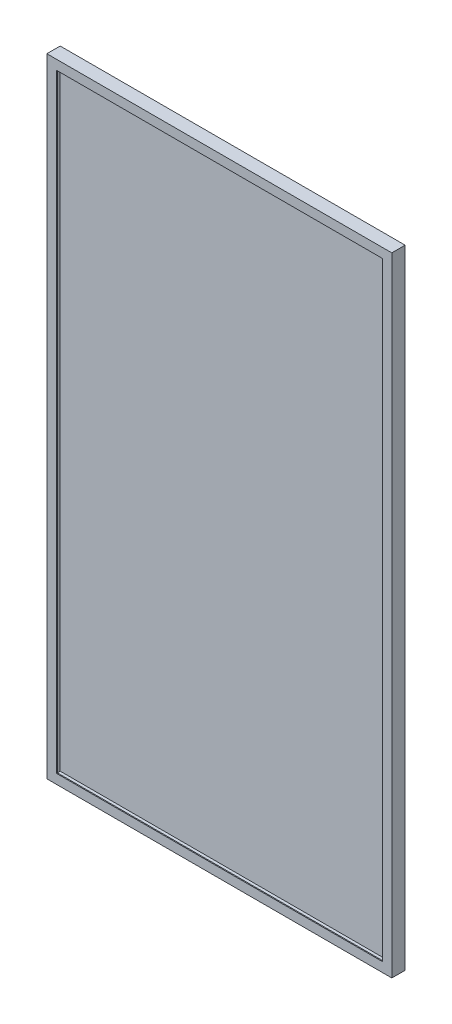
SolidWorks part; units mm, degrees
ref_plane "前视基准面" through (0, 0, 0) normal (0, 0, 1) x (1, 0, 0)
ref_plane "上视基准面" through (0, 0, 0) normal (0, 1, 0) x (1, 0, 0)
ref_plane "右视基准面" through (0, 0, 0) normal (1, 0, 0) x (0, 0, -1)
sketch "草图1" plane through (0, 0, 0) normal (0, 0, 1) x (1, 0, 0)
  line L1 (0, 0) -> (724.5, 0)
  line L2 (0, 0) -> (0, 1319)
  line L3 (0, 1319) -> (724.5, 1319)
  line L4 (724.5, 0) -> (724.5, 1319)
  dimension "D1" = 1319
  dimension "D2" = 724.5
extrude "凸台-拉伸1" add sketch "草图1" along normal blind 28
shell "抽壳1" thickness 2
sketch "草图2" plane through (0, 0, 28) normal (0, 0, 1) x (1, 0, 0)
  line L14 (20, 1299) -> (20, 20)
  line L15 (20, 20) -> (704.5, 20)
  line L16 (704.5, 20) -> (704.5, 1299)
  line L17 (704.5, 1299) -> (20, 1299)
  line L18 (20, 1299) -> (20, 20)
  line L19 (20, 20) -> (704.5, 20)
  line L20 (704.5, 20) -> (704.5, 1299)
  line L21 (704.5, 1299) -> (20, 1299)
  line L26 (0, 1319) -> (0, 0)
  line L27 (0, 0) -> (724.5, 0)
  line L28 (724.5, 0) -> (724.5, 1319)
  line L29 (724.5, 1319) -> (0, 1319)
  line L30 (0, 1319) -> (0, 0)
  line L31 (0, 0) -> (724.5, 0)
  line L32 (724.5, 0) -> (724.5, 1319)
  line L33 (724.5, 1319) -> (0, 1319)
  dimension "D1" = 20
  dimension "D2" = 0
extrude "凸台-拉伸2" add sketch "草图2" against normal blind 2
